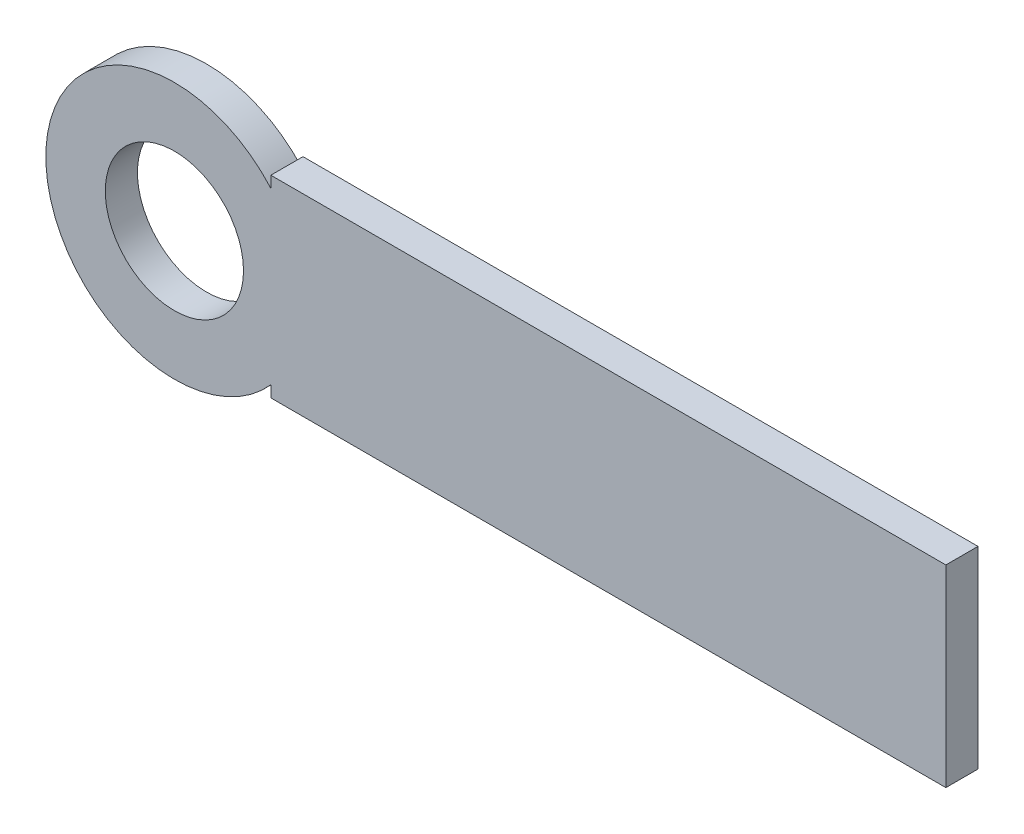
from build123d import *

# Parameters (mm, degrees)
SKETCH_1_R      = 4
SKETCH_1_R_2    = 2.15
EXTRUDE_1_DEPTH = 0.5
SKETCH_2_W      = 21
SKETCH_2_H      = 6
EXTRUDE_2_DEPTH = 0.5


with BuildPart() as part:
    # 草图1 → 凸台-拉伸1 (new, symmetric)
    with BuildSketch(Plane.XY):
        Circle(SKETCH_1_R)
        Circle(SKETCH_1_R_2, mode=Mode.SUBTRACT)
    extrude(amount=EXTRUDE_1_DEPTH, both=True)

    # 草图2 → 凸台-拉伸2 (add, symmetric)
    with BuildSketch(Plane.XY):
        with Locations((13.5, 0)):
            Rectangle(SKETCH_2_W, SKETCH_2_H)
    extrude(amount=EXTRUDE_2_DEPTH, both=True)


solid = part.part
